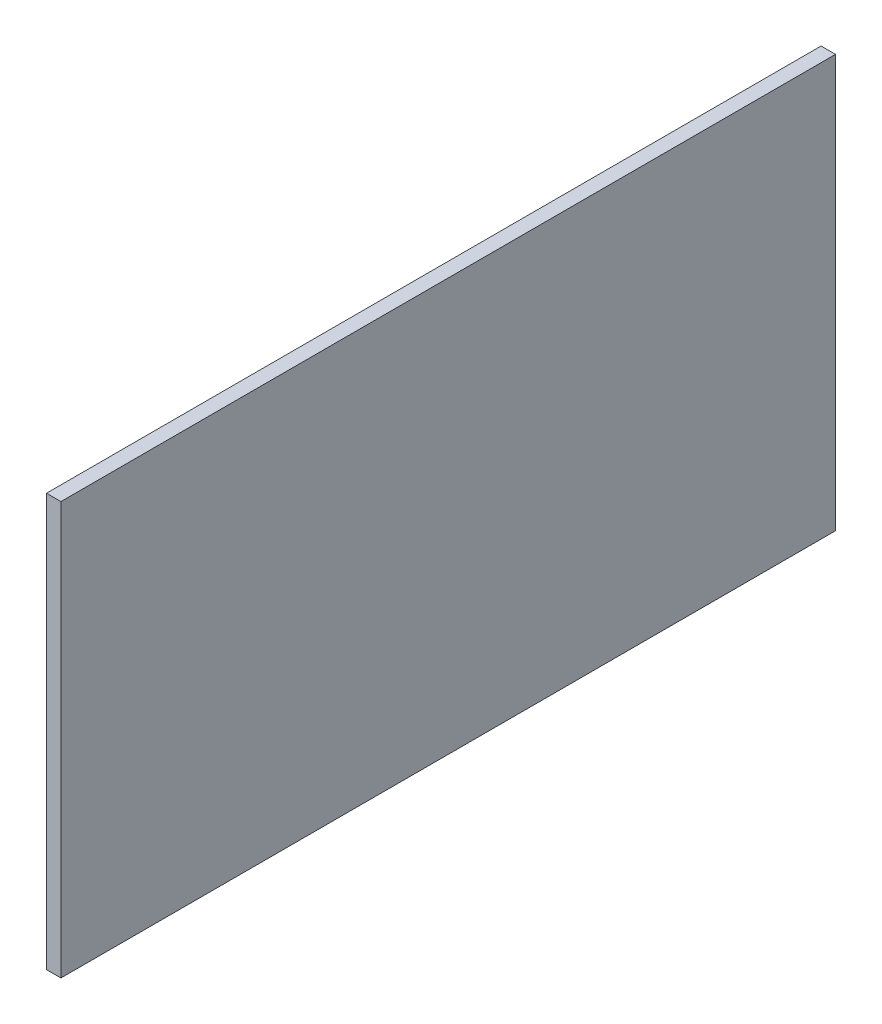
SolidWorks part; units mm, degrees
ref_plane "Front Plane" through (0, 0, 0) normal (0, 0, 1) x (1, 0, 0)
ref_plane "Top Plane" through (0, 0, 0) normal (0, 1, 0) x (1, 0, 0)
ref_plane "Right Plane" through (0, 0, 0) normal (1, 0, 0) x (0, 0, -1)
other "Configuration Table"
sketch "Sketch1" plane through (0, 0, 0) normal (1, 0, 0) x (0, 0, -1)
  line L1 (0, 0) -> (563.2, 0)
  line L2 (0, 0) -> (0, 300)
  line L3 (0, 300) -> (563.2, 300)
  line L4 (563.2, 0) -> (563.2, 300)
  dimension "D1" = 563.2
  dimension "D2" = 300
extrude "Boss-Extrude1" add sketch "Sketch1" along normal blind 10.5
